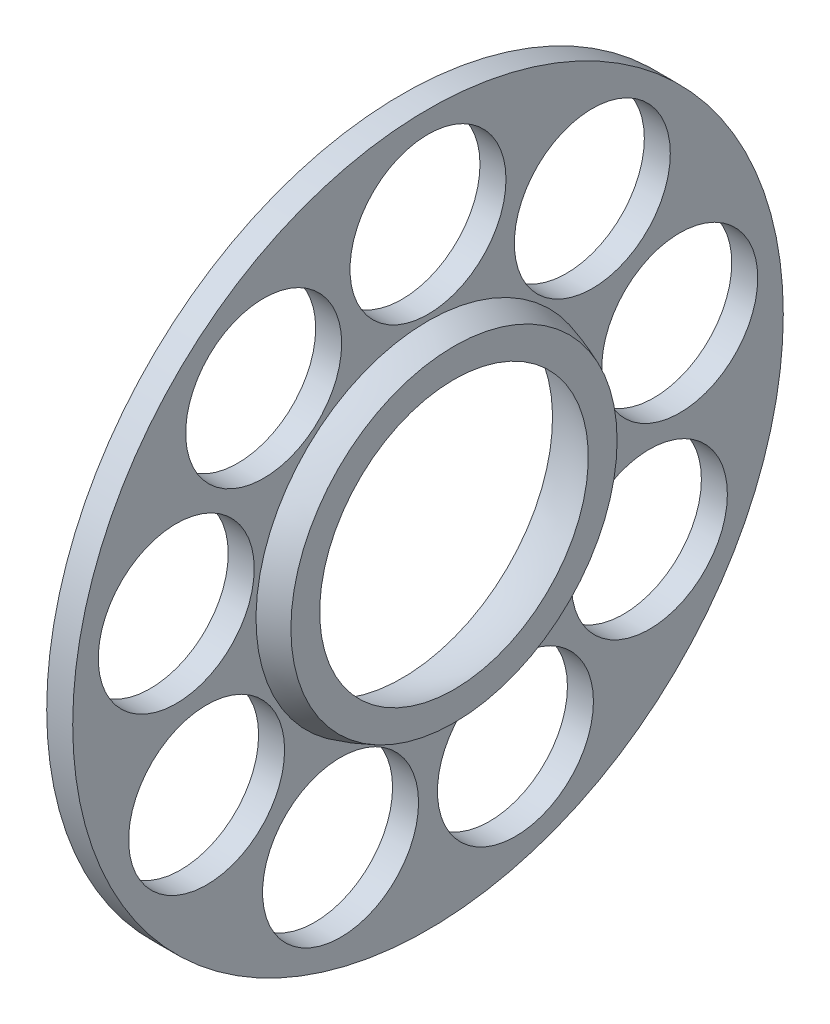
SolidWorks part; units mm, degrees
ref_plane "Front Plane" through (0, 0, 0) normal (0, 0, 1) x (1, 0, 0)
ref_plane "Top Plane" through (0, 0, 0) normal (0, 1, 0) x (1, 0, 0)
ref_plane "Right Plane" through (0, 0, 0) normal (1, 0, 0) x (0, 0, -1)
sketch "Sketch2" plane through (0, 0, 0) normal (0, 0, 1) x (1, 0, 0)
  line L0 (0, 0) -> (6, 0) construction
  line L1 (6, 0) -> (6, 18.8215)
  line L2 (0, 0) -> (-2.124, 0) construction
  line L3 (3, 19.8493) -> (3, 41)
  line L4 (3, 41) -> (0, 41)
  line L5 (0, 41) -> (0, 0)
  line L6 (6, 0) -> (0, 0)
  arc A0 (6, 15.5) -> (0, 17.3706) centre (-2.124, 0) ccw construction
  arc A1 (6, 18.8215) -> (3, 19.8493) centre (-2.124, 0) ccw
  arc A2 (4.1905, 19.5032) -> (-3.4994, 20.4538) centre (-2.124, 0) ccw construction
  arc A3 (3.2664, 16.6491) -> (-3.2981, 17.4606) centre (-2.124, 0) ccw construction
  point P5 (6, 15.5)
  dimension "D1" = 6
  dimension "D4" = 35
  dimension "D2" = 41
  dimension "D3" = 3
  dimension "D5" = 31
  dimension "D6" = 3
revolve "Revolve1" add sketch "Sketch2" angle 360 about L0
sketch "Sketch3" plane through (0, 0, 0) normal (0, 0, 1) x (1, 0, 0)
  line L0 (6, 15.5) -> (6, 0)
  line L1 (6, 0) -> (0, 0)
  line L2 (0, 0) -> (0, 17.3706)
  arc A0 (6, 15.5) -> (0, 17.3706) centre (-2.124, 0) ccw construction
  arc A1 (6, 15.5) -> (0, 17.3706) centre (-2.124, 0) ccw
revolve "Cut-Revolve1" cut sketch "Sketch3" angle 360 about L1
sketch "Sketch4" plane through (3, 0, 0) normal (1, 0, 0) x (0, 0, -1)
  line L0 (0, 0) -> (0, 29.5) construction
  circle A0 centre (0, 0) radius 29.5 construction
  circle A1 centre (0, 29.5) radius 9
  circle A2 centre (18.9622, 22.5983) radius 9
  circle A3 centre (29.0518, 5.1226) radius 9
  circle A4 centre (25.5477, -14.75) radius 9
  circle A5 centre (10.0896, -27.7209) radius 9
  circle A6 centre (-10.0896, -27.7209) radius 9
  circle A7 centre (-25.5477, -14.75) radius 9
  circle A8 centre (-29.0518, 5.1226) radius 9
  circle A9 centre (-18.9622, 22.5983) radius 9
  point P24 (0, 0)
  dimension "D1" = 59
  dimension "D2" = 18
  dimension "D3" = 9
extrude "Cut-Extrude1" cut sketch "Sketch4" against normal blind 10
